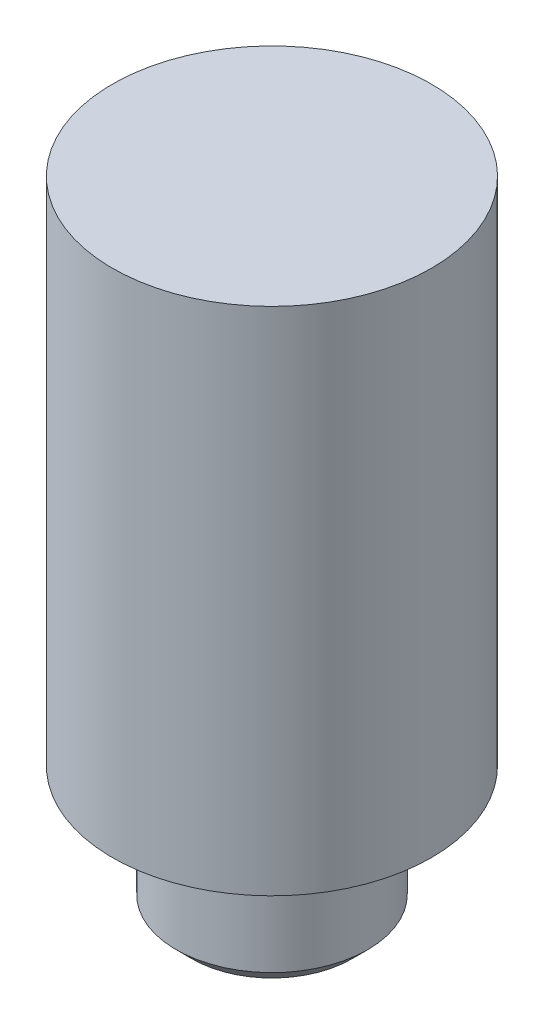
SolidWorks part; units mm, degrees
material "Plain Carbon Steel"
ref_plane "Front Plane" through (0, 0, 0) normal (0, 0, 1) x (1, 0, 0)
ref_plane "Top Plane" through (0, 0, 0) normal (0, 1, 0) x (1, 0, 0)
ref_plane "Right Plane" through (0, 0, 0) normal (1, 0, 0) x (0, 0, -1)
sketch "Sketch1" plane through (0, 0, 0) normal (0, 0, 1) x (1, 0, 0)
  line L0 (0, -324.9645) -> (0, 15923.2606) construction
  line L1 (0, 0) -> (5, 0)
  line L2 (5, 0) -> (5, -16)
  line L3 (5, -16) -> (3, -16)
  line L4 (3, -16) -> (3, -20)
  line L5 (3, -20) -> (0, -20)
  line L6 (0, -20) -> (0, 0)
  dimension "D1" = 5
  dimension "D2" = 3
  dimension "D3" = 16
  dimension "D4" = 20
revolve "Revolve1" add sketch "Sketch1" angle 360 about L0
chamfer "Chamfer2" distance 0.5 angle 45 1 edges at (3, -20, 0)
